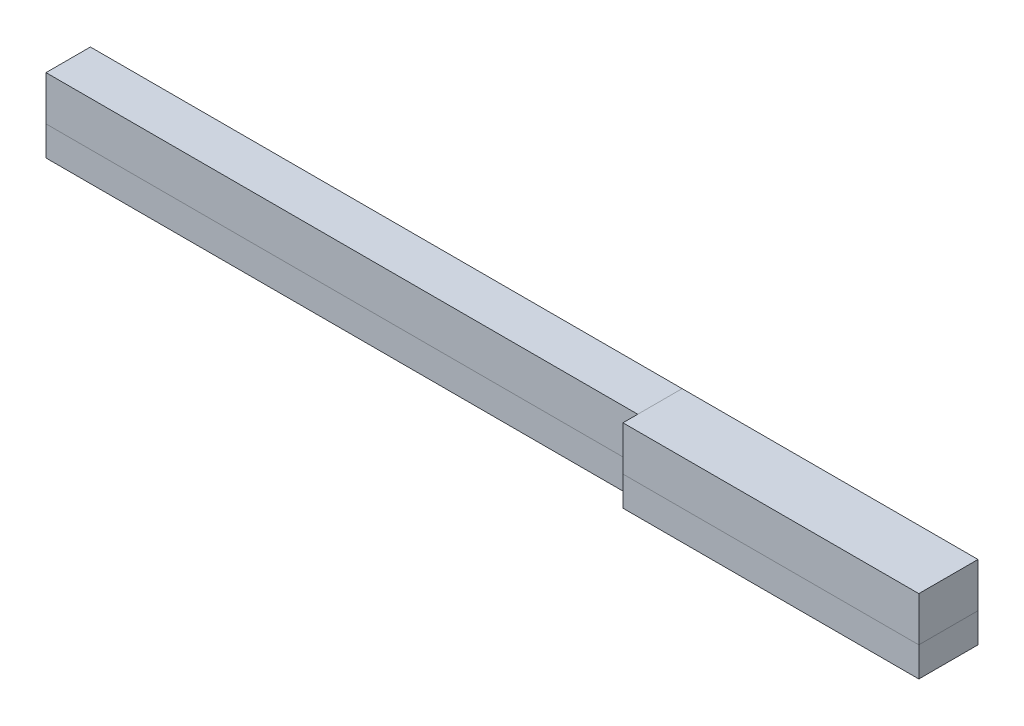
from build123d import *

# Parameters (mm, degrees)
SKETCH_1_W      = 20
SKETCH_1_H      = 4
EXTRUDE_1_DEPTH = 2
SKETCH_3_W      = 20
SKETCH_3_H      = 4
EXTRUDE_2_DEPTH = 3
SKETCH_4_W      = 40
SKETCH_4_H      = 3
EXTRUDE_3_DEPTH = 2
SKETCH_5_W      = 40
SKETCH_5_H      = 3
EXTRUDE_4_DEPTH = 3


with BuildPart() as part:
    # 草图1 → 凸台-拉伸1 (new body)
    with BuildSketch(Plane(origin=(0, 0, 0), x_dir=(1, 0, 0), z_dir=(0, 1, 0))):
        Rectangle(SKETCH_1_W, SKETCH_1_H)
    extrude(amount=EXTRUDE_1_DEPTH)


with BuildPart() as body_2:
    # 草图3 → 凸台-拉伸2 (new body)
    with BuildSketch(Plane(origin=(0, 2, 0), x_dir=(1, 0, 0), z_dir=(0, 1, 0))):
        Rectangle(SKETCH_3_W, SKETCH_3_H)
    extrude(amount=EXTRUDE_2_DEPTH)


with BuildPart() as body_3:
    # 草图4 → 凸台-拉伸3 (new body)
    with BuildSketch(Plane.XZ):
        with Locations((-30, -0.5)):
            Rectangle(SKETCH_4_W, SKETCH_4_H)
    extrude(amount=-EXTRUDE_3_DEPTH)


with BuildPart() as body_4:
    # 草图5 → 凸台-拉伸4 (new body)
    with BuildSketch(Plane(origin=(0, 2, 0), x_dir=(1, 0, 0), z_dir=(0, 1, 0))):
        with Locations((-30, 0.5)):
            Rectangle(SKETCH_5_W, SKETCH_5_H)
    extrude(amount=EXTRUDE_4_DEPTH)


solid = Compound([part.part, body_2.part, body_3.part, body_4.part])
